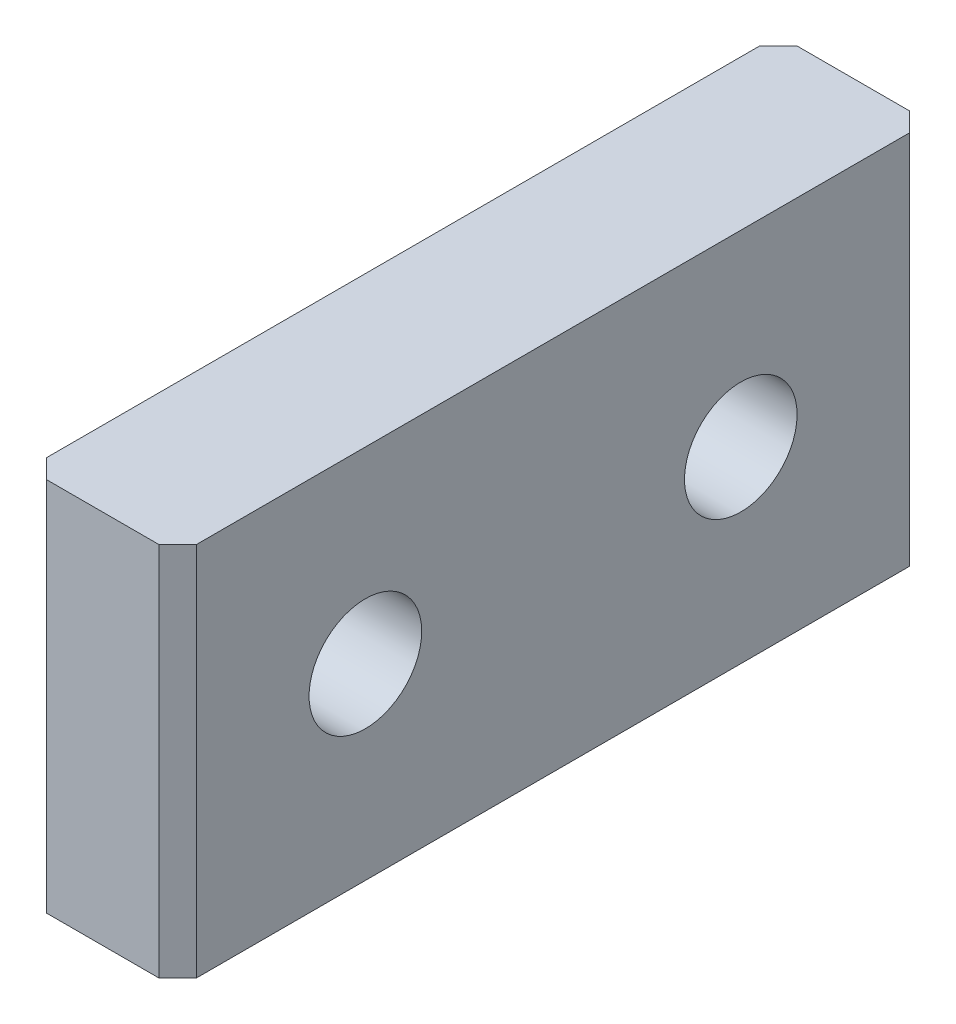
from build123d import *

# Parameters (mm, degrees)
SKETCH1_W           = 8
SKETCH1_H           = 40
BOSS_EXTRUDE1_DEPTH = 20
CHAMFER1_SIZE       = 1
SKETCH2_R           = 3
CUT_EXTRUDE1_DEPTH  = 46.431266766


with BuildPart() as part:
    # Sketch1 → Boss-Extrude1 (new body)
    with BuildSketch(Plane(origin=(0, 0, 0), x_dir=(1, 0, 0), z_dir=(0, 1, 0))):
        with Locations((4, -20)):
            Rectangle(SKETCH1_W, SKETCH1_H)
    extrude(amount=BOSS_EXTRUDE1_DEPTH)

    # Chamfer1
    chamfer1_edges = [part.edges().sort_by_distance(p)[0] for p in [
        (0, 10, 0),
        (8, 10, 0),
        (8, 10, 40),
        (0, 10, 40),
    ]]
    chamfer(chamfer1_edges, length=CHAMFER1_SIZE)

    # Sketch2 → Cut-Extrude1 (cut, through all)
    with BuildSketch(Plane(origin=(8, 0, 0), x_dir=(0, 0, -1), z_dir=(1, 0, 0))):
        with Locations((-30, 10)):
            Circle(SKETCH2_R)
        with Locations((-10, 10)):
            Circle(SKETCH2_R)
    extrude(amount=-CUT_EXTRUDE1_DEPTH, mode=Mode.SUBTRACT)


solid = part.part
